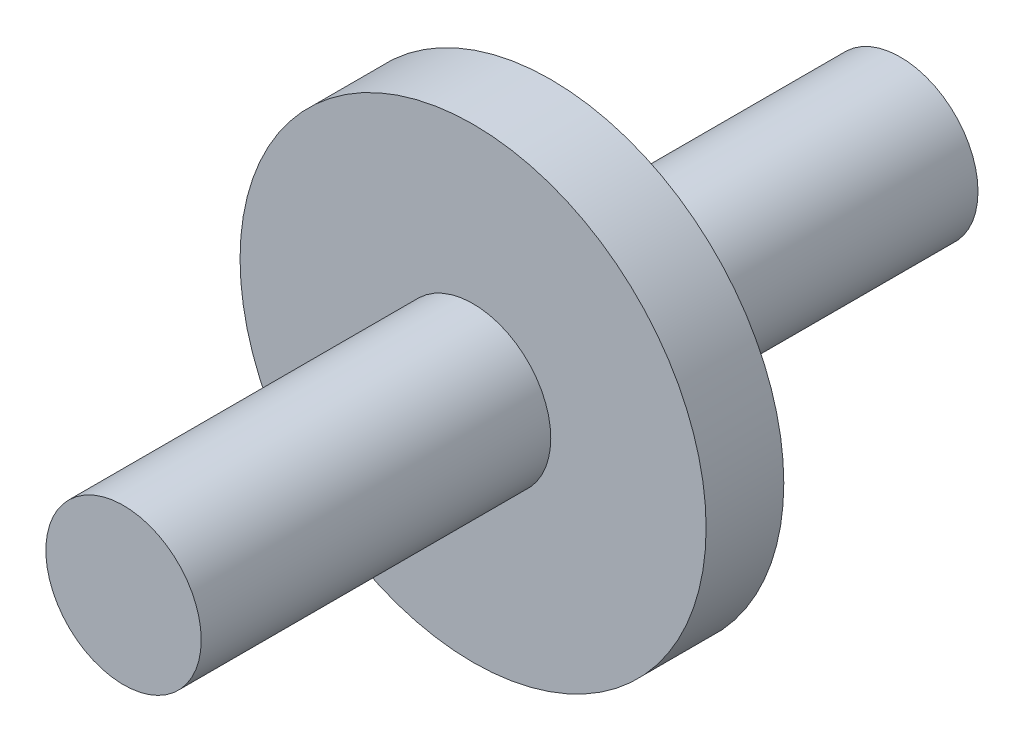
from build123d import *

# Parameters (mm, degrees)
SKETCH1_R           = 40
BOSS_EXTRUDE1_DEPTH = 200
SKETCH2_R           = 120
BOSS_EXTRUDE2_DEPTH = 20


with BuildPart() as part:
    # Sketch1 → Boss-Extrude1 (new, symmetric)
    with BuildSketch(Plane.XY):
        Circle(SKETCH1_R)
    extrude(amount=BOSS_EXTRUDE1_DEPTH, both=True)

    # Sketch2 → Boss-Extrude2 (add, symmetric)
    with BuildSketch(Plane.XY):
        Circle(SKETCH2_R)
    extrude(amount=BOSS_EXTRUDE2_DEPTH, both=True)


solid = part.part
